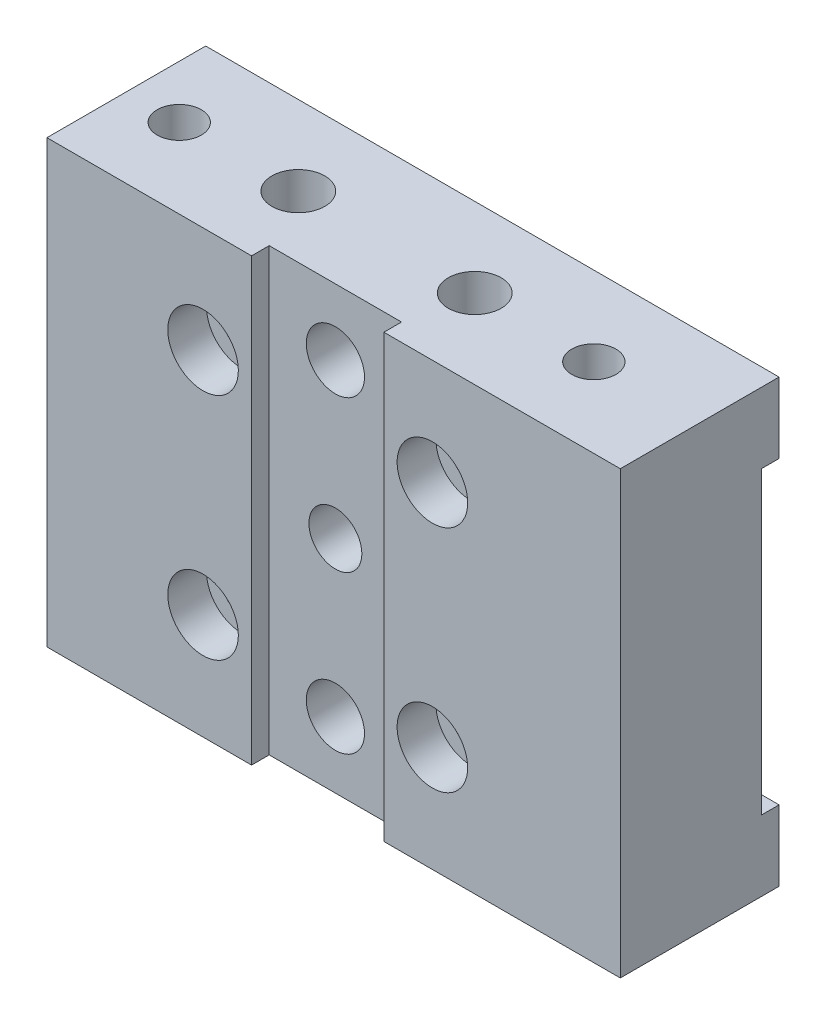
from build123d import *

# Parameters (mm, degrees)
SKETCH_1_W                   = 65
SKETCH_1_H                   = 50
EXTRUDE_1_DEPTH              = 9
SKETCH_4_W                   = 2
SKETCH_4_H                   = 34
CUT_EXTRUDE_1_DEPTH          = 71.221079456
HOLE_WIZARD_M4_1_D           = 4.5
HOLE_WIZARD_M4_1_CBORE_D     = 8
HOLE_WIZARD_M4_1_CBORE_DEPTH = 4.4
SKETCH_8_W                   = 15
SKETCH_8_H                   = 50
CUT_EXTRUDE_3_DEPTH          = 2
F_6_0MM_1_D                  = 6
F_6_0MM_1_DEPTH              = 7
F_6_0MM_1_TIP                = 1.802581857
HOLE_WIZARD_M6_2_D           = 6.6
HOLE_WIZARD_M6_2_CBORE_D     = 11
HOLE_WIZARD_M6_2_CBORE_DEPTH = 9
HOLE_WIZARD_M6_1_D           = 5
HOLE_WIZARD_M6_1_DEPTH       = 15
HOLE_WIZARD_M6_1_TIP         = 1.502151548
F_6_0MM_2_D                  = 6
F_6_0MM_2_DEPTH              = 6
F_6_0MM_2_TIP                = 1.802581857


with BuildPart() as part:
    # 草图1 → 凸台-拉伸1 (new, symmetric)
    with BuildSketch(Plane.XY):
        Rectangle(SKETCH_1_W, SKETCH_1_H)
    extrude(amount=EXTRUDE_1_DEPTH, both=True)

    # 草图4 → 切除-拉伸1 (cut, through all)
    with BuildSketch(Plane(origin=(32.5, 0, 0), x_dir=(0, 0, -1), z_dir=(1, 0, 0))):
        with Locations((8, 0)):
            Rectangle(SKETCH_4_W, SKETCH_4_H)
    extrude(amount=-CUT_EXTRUDE_1_DEPTH, mode=Mode.SUBTRACT)

    # Hole Wizard M4 _1 (through all)
    with Locations(Plane.XY.offset(9)):
        with Locations((11.2, -13), (-14.8, -13), (-14.8, 13), (11.2, 13)):
            CounterBoreHole(HOLE_WIZARD_M4_1_D / 2, HOLE_WIZARD_M4_1_CBORE_D / 2, HOLE_WIZARD_M4_1_CBORE_DEPTH)

    # 草图8 → 切除-拉伸3 (cut)
    with BuildSketch(Plane.XY.offset(9)):
        with Locations((-1.8, 0)):
            Rectangle(SKETCH_8_W, SKETCH_8_H)
    extrude(amount=-CUT_EXTRUDE_3_DEPTH, mode=Mode.SUBTRACT)

    # Ø6.0mm 暗销孔1
    with Locations(Plane.XY.offset(7)):
        with Locations((-1.8, 0)):
            Hole(F_6_0MM_1_D / 2, depth=F_6_0MM_1_DEPTH)
            with Locations((0, 0, -(F_6_0MM_1_DEPTH + F_6_0MM_1_TIP / 2))):  # 118° drill point
                Cone(0, F_6_0MM_1_D / 2, F_6_0MM_1_TIP, mode=Mode.SUBTRACT)

    # M6 六角凹头螺钉的柱形沉头孔2 (through all)
    with Locations(Plane(origin=(0, 0, -9), x_dir=(-1, 0, 0), z_dir=(0, 0, -1))):
        with Locations((1.8, 17.5), (1.8, -17.5)):
            CounterBoreHole(HOLE_WIZARD_M6_2_D / 2, HOLE_WIZARD_M6_2_CBORE_D / 2, HOLE_WIZARD_M6_2_CBORE_DEPTH)

    # M6 螺纹孔1
    with Locations(Plane(origin=(0, 25, 0), x_dir=(1, 0, 0), z_dir=(0, 1, 0))):
        with Locations((20.5, 0), (-26.5, 0)):
            Hole(HOLE_WIZARD_M6_1_D / 2, depth=HOLE_WIZARD_M6_1_DEPTH)
            with Locations((0, 0, -(HOLE_WIZARD_M6_1_DEPTH + HOLE_WIZARD_M6_1_TIP / 2))):  # 118° drill point
                Cone(0, HOLE_WIZARD_M6_1_D / 2, HOLE_WIZARD_M6_1_TIP, mode=Mode.SUBTRACT)

    # Ø6.0mm 暗销孔2
    with Locations(Plane(origin=(0, 25, 0), x_dir=(1, 0, 0), z_dir=(0, 1, 0))):
        with Locations((7, 0), (-13, 0)):
            Hole(F_6_0MM_2_D / 2, depth=F_6_0MM_2_DEPTH)
            with Locations((0, 0, -(F_6_0MM_2_DEPTH + F_6_0MM_2_TIP / 2))):  # 118° drill point
                Cone(0, F_6_0MM_2_D / 2, F_6_0MM_2_TIP, mode=Mode.SUBTRACT)


solid = part.part
